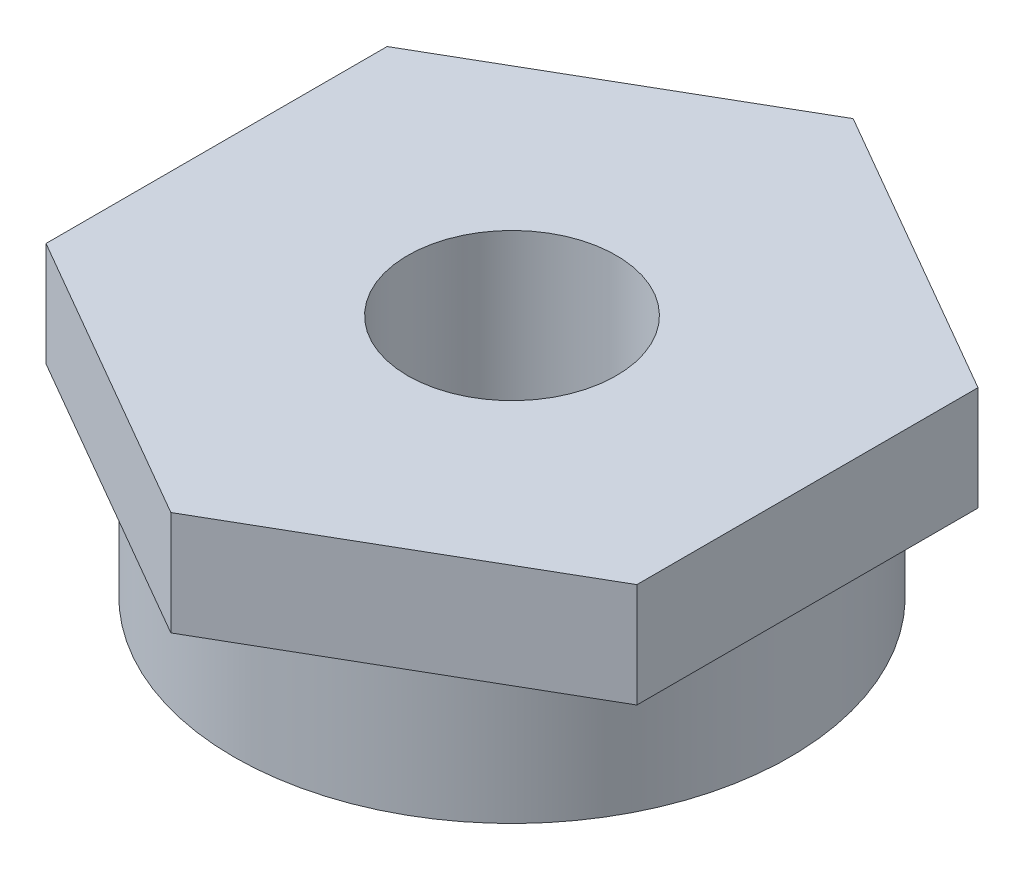
from build123d import *

# Parameters (mm, degrees)
SKETCH1_R           = 4
BOSS_EXTRUDE1_DEPTH = 2
BOSS_EXTRUDE2_DEPTH = 1.5
SKETCH3_R           = 1.5
CUT_EXTRUDE1_DEPTH  = 8.375353099


with BuildPart() as part:
    # Sketch1 → Boss-Extrude1 (new body)
    with BuildSketch(Plane(origin=(0, 0, 0), x_dir=(1, 0, 0), z_dir=(0, 1, 0))):
        with Locations(Location((0, 0, 0), (0, 0, 270))):
            Circle(SKETCH1_R)
    extrude(amount=BOSS_EXTRUDE1_DEPTH)

    # Sketch2 → Boss-Extrude2 (add)
    with BuildSketch(Plane(origin=(0, 2, 0), x_dir=(1, 0, 0), z_dir=(0, 1, 0))):
        Polygon((0, 4.907477288), (-4.25, 2.453738644), (-4.25, -2.453738644), (0, -4.907477288), (4.25, -2.453738644), (4.25, 2.453738644), align=None)
    extrude(amount=BOSS_EXTRUDE2_DEPTH)

    # Sketch3 → Cut-Extrude1 (cut, through all)
    with BuildSketch(Plane(origin=(0, 3.5, 0), x_dir=(1, 0, 0), z_dir=(0, 1, 0))):
        with Locations(Location((0, 0, 0), (0, 0, 270))):
            Circle(SKETCH3_R)
    extrude(amount=-CUT_EXTRUDE1_DEPTH, mode=Mode.SUBTRACT)


solid = part.part
